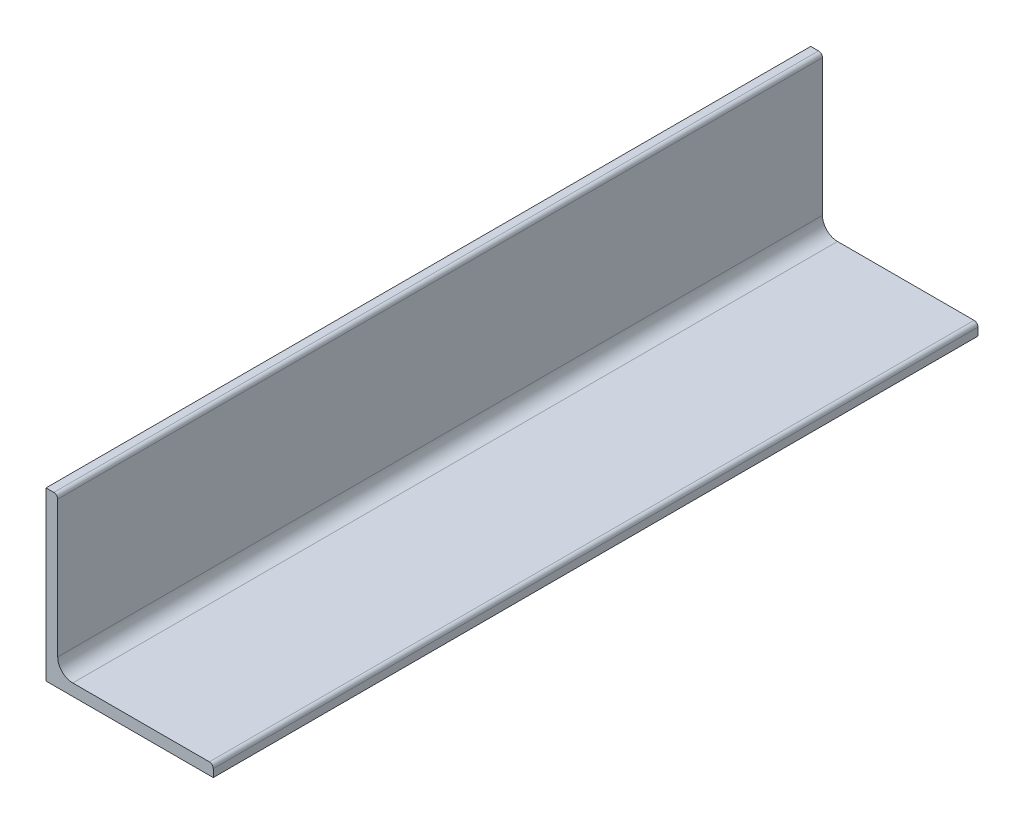
SolidWorks part; units mm, degrees
material "普通碳钢"
ref_plane "Front Plane" through (0, 0, 0) normal (0, 0, 1) x (1, 0, 0)
ref_plane "Top Plane" through (0, 0, 0) normal (0, 1, 0) x (1, 0, 0)
ref_plane "Right Plane" through (0, 0, 0) normal (1, 0, 0) x (0, 0, -1)
sketch "Sketch1" plane through (0, 0, 0) normal (0, 0, 1) x (1, 0, 0)
  line L0 (0, 200) -> (0, 0)
  line L1 (0, 0) -> (200, 0)
  line L2 (14, 195.3333) -> (14, 32)
  line L3 (32, 14) -> (195.3333, 14)
  line L4 (0, 200) -> (9.3333, 200)
  line L5 (200, 0) -> (200, 9.3333)
  arc A0 (9.3333, 200) -> (14, 195.3333) centre (9.3333, 195.3333) cw
  arc A1 (200, 9.3333) -> (195.3333, 14) centre (195.3333, 9.3333) ccw
  arc A2 (14, 32) -> (32, 14) centre (32, 32) ccw
  dimension "D4" = 4.6667
  dimension "D5" = 18
  dimension "D1" = 200
  dimension "D2" = 14
  dimension "D3" = 14
  dimension "D6" = 0
  dimension "D7" = 0
extrude "Boss-Extrude1" add sketch "Sketch1" along normal mid plane 914.4
